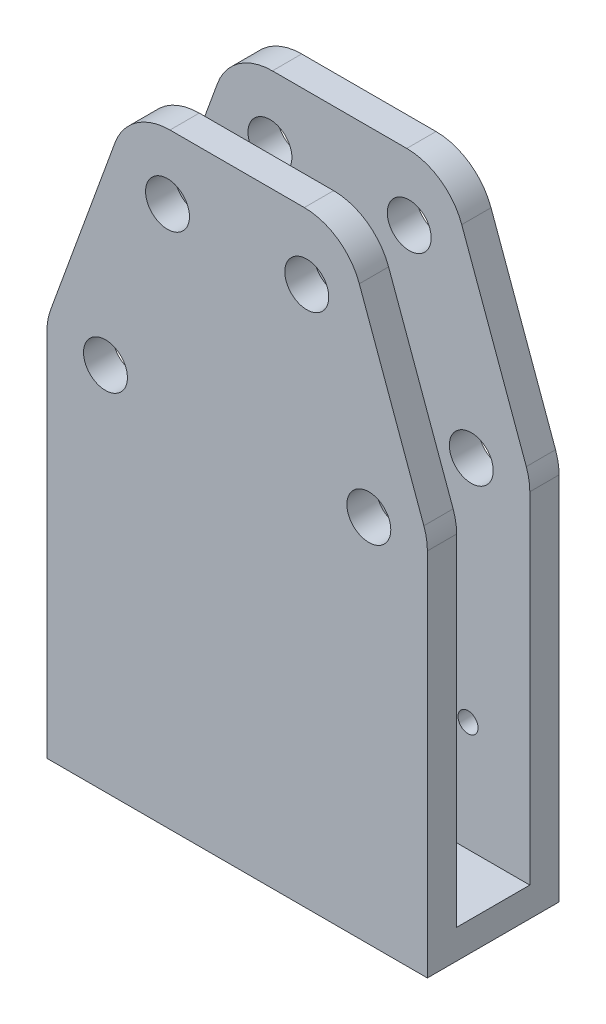
SolidWorks part; units mm, degrees
ref_plane "Front Plane" through (0, 0, 0) normal (0, 0, 1) x (1, 0, 0)
ref_plane "Top Plane" through (0, 0, 0) normal (0, 1, 0) x (1, 0, 0)
ref_plane "Right Plane" through (0, 0, 0) normal (1, 0, 0) x (0, 0, -1)
ref_plane "Plane1" through (0, 0, 10) normal (0, 0, 1) x (1, 0, 0)
sketch "Sketch1" plane through (0, 0, 10) normal (0, 0, 1) x (1, 0, 0)
  line L0 (-65, 200) -> (-65, 70.0932)
  line L1 (-65, 70.0932) -> (65, 70.0932)
  line L2 (65, 70.0932) -> (65, 200)
  line L3 (65, 200) -> (36.9543, 277.0548)
  line L4 (36.9543, 277.0548) -> (-36.9543, 277.0548)
  line L5 (-36.9543, 277.0548) -> (-65, 200)
  dimension "D1" = 28.0457
  dimension "D2" = 101.9543
  dimension "D3" = 130
  dimension "D4" = 129.9068
  dimension "D5" = 206.9616
extrude "Boss-Extrude1" add sketch "Sketch1" against normal blind 10
sketch "Sketch2" plane through (0, 0, 10) normal (0, 0, 1) x (1, 0, 0)
  line L0 (-65, 70.0932) -> (-65, 80.0932)
  line L1 (-65, 80.0932) -> (65, 80.0932)
  line L2 (65, 80.0932) -> (65, 70.0932)
  line L3 (65, 70.0932) -> (-65, 70.0932)
  line L4 (-65, 200) -> (-65, 70.0932) construction
  line L5 (-65, 70.0932) -> (65, 70.0932) construction
  dimension "D1" = 130
  dimension "D2" = 10
extrude "Boss-Extrude2" add sketch "Sketch2" along normal blind 25
sketch "Sketch3" plane through (0, 0, 35) normal (0, 0, 1) x (1, 0, 0)
  line L0 (-65, 70.0932) -> (-65, 200)
  line L1 (-65, 200) -> (-36.9543, 277.0548)
  line L2 (-36.9543, 277.0548) -> (36.9543, 277.0548)
  line L3 (36.9543, 277.0548) -> (65, 200)
  line L4 (65, 200) -> (65, 70.0932)
  line L5 (65, 70.0932) -> (-65, 70.0932)
  line L6 (65, 70.0932) -> (65, 80.0932) construction
  line L7 (-65, 70.0932) -> (65, 70.0932) construction
  dimension "D1" = 28.0457
  dimension "D2" = 101.9543
  dimension "D3" = 130
  dimension "D4" = 129.9068
  dimension "D5" = 206.9616
extrude "Boss-Extrude3" add sketch "Sketch3" along normal blind 10
sketch "Sketch4" plane through (0, 0, 35) normal (0, 0, -1) x (-1, 0, 0)
  line L0 (-18.0453, 207.0548) -> (18.0453, 207.0548)
  line L1 (22.7438, 213.7649) -> (12.4471, 242.0548)
  line L2 (12.4471, 242.0548) -> (-12.4471, 242.0548)
  line L3 (-12.4471, 242.0548) -> (-22.7438, 213.7649)
  line L4 (65, 200) -> (65, 80.0932) construction
  line L5 (-65, 80.0932) -> (65, 80.0932) construction
  arc A0 (-22.7438, 213.7649) -> (-18.0453, 207.0548) centre (-18.0453, 212.0548) ccw
  arc A1 (18.0453, 207.0548) -> (22.7438, 213.7649) centre (18.0453, 212.0548) ccw
  dimension "D1" = 5
  dimension "D2" = 42.2562
  dimension "D3" = 46.9547
  dimension "D4" = 52.5529
  dimension "D5" = 77.4471
  dimension "D6" = 126.9616
extrude "Cut-Extrude1" cut sketch "Sketch4" against normal blind 5
sketch "Sketch5" plane through (0, 0, 10) normal (0, 0, 1) x (1, 0, 0)
  line L0 (22.7438, 213.7649) -> (12.4471, 242.0548)
  line L1 (12.4471, 242.0548) -> (-12.4471, 242.0548)
  line L2 (-12.4471, 242.0548) -> (-22.7438, 213.7649)
  line L3 (-18.0453, 207.0548) -> (18.0453, 207.0548)
  line L4 (65, 80.0932) -> (65, 200) construction
  line L5 (65, 80.0932) -> (-65, 80.0932) construction
  arc A0 (-22.7438, 213.7649) -> (-18.0453, 207.0548) centre (-18.0453, 212.0548) ccw
  arc A1 (18.0453, 207.0548) -> (22.7438, 213.7649) centre (18.0453, 212.0548) ccw
  dimension "D1" = 5
  dimension "D2" = 42.2562
  dimension "D3" = 46.9547
  dimension "D4" = 52.5529
  dimension "D5" = 77.4471
  dimension "D6" = 126.9616
extrude "Cut-Extrude2" cut sketch "Sketch5" against normal blind 5
hole_wizard "Ø15.0 (15) Diameter Hole1" positions "Sketch7" profile "Sketch6" hole size "Ø15.0" standard "ANSI Metric"
sketch "Sketch7" plane through (0, 0, 45) normal (0, 0, 1) x (1, 0, 0)
  point P0 (8.8889, 130.7392)
  point P1 (45, 196.4735)
  point P2 (-45, 196.4735)
  point P3 (-23.7948, 254.7344)
  point P4 (23.7948, 254.7344)
sketch "Sketch6" plane through (8.8889, 130.7392, 45) normal (1, 0, 0) x (0, -1, 0)
  line L0 (0, 0) -> (0, 10)
  line L1 (0, 10) -> (7.5, 10)
  line L2 (7.5, 10) -> (7.5, 0)
  line L5 (7.5, 0) -> (0, 0)
  line L11 (0, -6.35) -> (0, 107.95) construction
  dimension "通孔孔直径" = 15
  dimension "通孔孔深度" = 10
hole_wizard "Hole1" positions "Sketch9" profile "Sketch8" legacy
sketch "Sketch9" plane through (0, 0, 45) normal (0, 0, 1) x (1, 0, 0)
  point P0 (-9.3119, 122.4487)
  point P1 (0.5984, 148.94)
  point P2 (27.0896, 139.0297)
  point P3 (17.1794, 112.5385)
sketch "Sketch8" plane through (-9.3119, 122.4487, 45) normal (1, 0, 0) x (0, -1, 0)
  line L0 (0, 0) -> (0, 10)
  line L1 (0, 10) -> (2.5941, 10)
  line L2 (2.5941, 10) -> (2.5941, 0)
  line L3 (2.5941, 0) -> (0, 0)
  line L4 (0, 110) -> (0, -10) construction
  dimension "直径" = 5.1881
  dimension "深度" = 10
hole_wizard "Ø15.0 (15) Diameter Hole2" positions "Sketch11" profile "Sketch10" hole size "Ø15.0" standard "ANSI Metric"
sketch "Sketch11" plane through (0, 0, 0) normal (0, 0, -1) x (-1, 0, 0)
  point P0 (-8.8889, 130.7392)
  point P1 (-45, 196.4735)
  point P2 (45, 196.4735)
  point P3 (23.7948, 254.7344)
  point P4 (-23.7948, 254.7344)
sketch "Sketch10" plane through (8.8889, 130.7392, 0) normal (1, 0, 0) x (0, 1, 0)
  line L0 (0, 0) -> (0, 45)
  line L1 (0, 45) -> (7.5, 45)
  line L2 (7.5, 45) -> (7.5, 0)
  line L5 (7.5, 0) -> (0, 0)
  line L11 (0, -6.35) -> (0, 107.95) construction
  dimension "通孔孔直径" = 15
  dimension "通孔孔深度" = 45
fillet "Fillet1" radius 5 4 edges at (-12.4471, 242.0548, 7.5) (12.4471, 242.0548, 7.5) (12.4471, 242.0548, 37.5) (-12.4471, 242.0548, 37.5)
fillet "Fillet2" radius 20 8 edges at (-65, 200, 40) (36.9543, 277.0548, 40) (65, 200, 40) (-36.9543, 277.0548, 5) (-36.9543, 277.0548, 40) (65, 200, 5) (-65, 200, 5) (36.9543, 277.0548, 5)
scale "Scale1" scale about origin uniform scaling yes scale factor 0.3
sketch "Sketch14" plane through (0, 0, 13.5) normal (0, 0, 1) x (1, 0, 0)
  line L1 (-7.5047, 30.0623) -> (11.843, 30.0623)
  line L2 (-7.5047, 30.0623) -> (-7.5047, 46.4889)
  line L3 (-7.5047, 46.4889) -> (11.843, 46.4889)
  line L4 (11.843, 30.0623) -> (11.843, 46.4889)
extrude "Boss-Extrude4" add sketch "Sketch14" against normal up to surface (3 mm away) up to face at (-3.5718, 36.7346, 10.5)
hole_wizard "M2.5 Tapped Hole1" positions "Sketch16" profile "Sketch17" tap size "M2.5" standard "GB"
sketch "Sketch16" plane through (0, 0, 0) normal (0, 0, -1) x (-1, 0, 0)
  point P2 (7.8333, 35.3218)
  point P4 (-13.1667, 35.3218)
sketch "Sketch17" plane through (-7.8333, 35.3218, 0) normal (1, 0, 0) x (0, 1, 0)
  line L0 (0, 0) -> (0, 6.9659)
  line L1 (0, 6.9659) -> (1.025, 6.35)
  line L2 (1.025, 6.35) -> (1.025, 0)
  line L5 (1.025, 0) -> (0, 0)
  line L10 (0, 6.9659) -> (-1.025, 6.35) construction
  line L11 (0, -6.35) -> (0, 107.95) construction
  dimension "螺纹孔钻头直径" = 2.05
  dimension "螺纹孔钻头深度" = 6.35
  dimension "导头角度" = 118
cosmetic thread "Cosmetic Thread1" parameters "D1"=3, "D2"=2.5
cosmetic thread "Cosmetic Thread2" parameters "D1"=3, "D2"=2.5
hole_wizard "M5 Tapped Hole1" positions "Sketch18" profile "Sketch19" tap size "M5" standard "GB" end condition through all
sketch "Sketch18" plane through (0, 21.028, 0) normal (0, -1, 0) x (-1, 0, 0)
  line L0 (0, 0) -> (0, -20.5808) construction
  line L3 (19.5, -6.75) -> (-23.5269, -6.75) construction
  line L4 (19.5, 0) -> (19.5, -13.5) construction
  point P0 (12.5, -6.75)
  point P18 (-12.5, -6.75)
  dimension "D1" = 12.5
sketch "Sketch19" plane through (-12.5, 21.028, 6.75) normal (1, 0, 0) x (0, 0, -1)
  line L0 (0, 0) -> (0, 62.0885)
  line L1 (0, 62.0885) -> (2.1, 62.0885)
  line L2 (2.1, 62.0885) -> (2.1, 0)
  line L5 (2.1, 0) -> (0, 0)
  line L11 (0, -6.35) -> (0, 107.95) construction
  dimension "通孔螺纹孔钻头直径" = 4.2
  dimension "通孔螺纹孔钻头深度" = 62.0885
cosmetic thread "Cosmetic Thread3" parameters "D2"=5
cosmetic thread "Cosmetic Thread4" parameters "D2"=5
